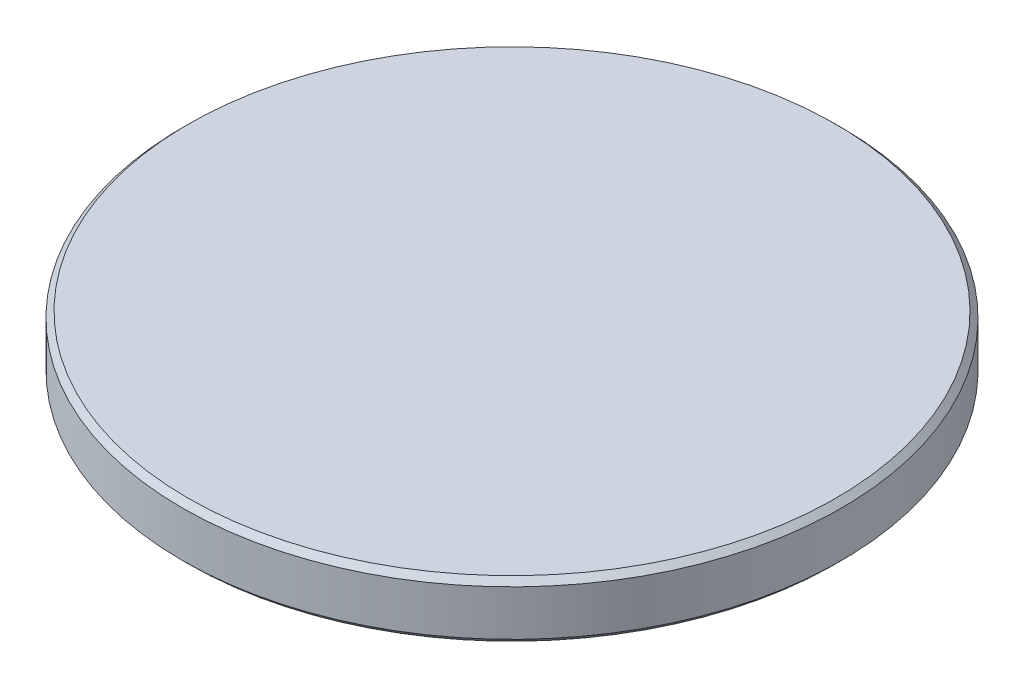
from build123d import *

# Parameters (mm, degrees)
SKETCH1_R           = 58
BOSS_EXTRUDE1_DEPTH = 10
CHAMFER1_SIZE       = 1


with BuildPart() as part:
    # Sketch1 → Boss-Extrude1 (new body)
    with BuildSketch(Plane(origin=(0, 0, 0), x_dir=(1, 0, 0), z_dir=(0, 1, 0))):
        with Locations(Location((0, 0, 0), (0, 0, 270))):
            Circle(SKETCH1_R)
    extrude(amount=BOSS_EXTRUDE1_DEPTH)

    # Chamfer1
    chamfer1_edges = [part.edges().sort_by_distance(p)[0] for p in [
        (0, 0, -58),
        (0, 10, -58),
    ]]
    chamfer(chamfer1_edges, length=CHAMFER1_SIZE)


solid = part.part
